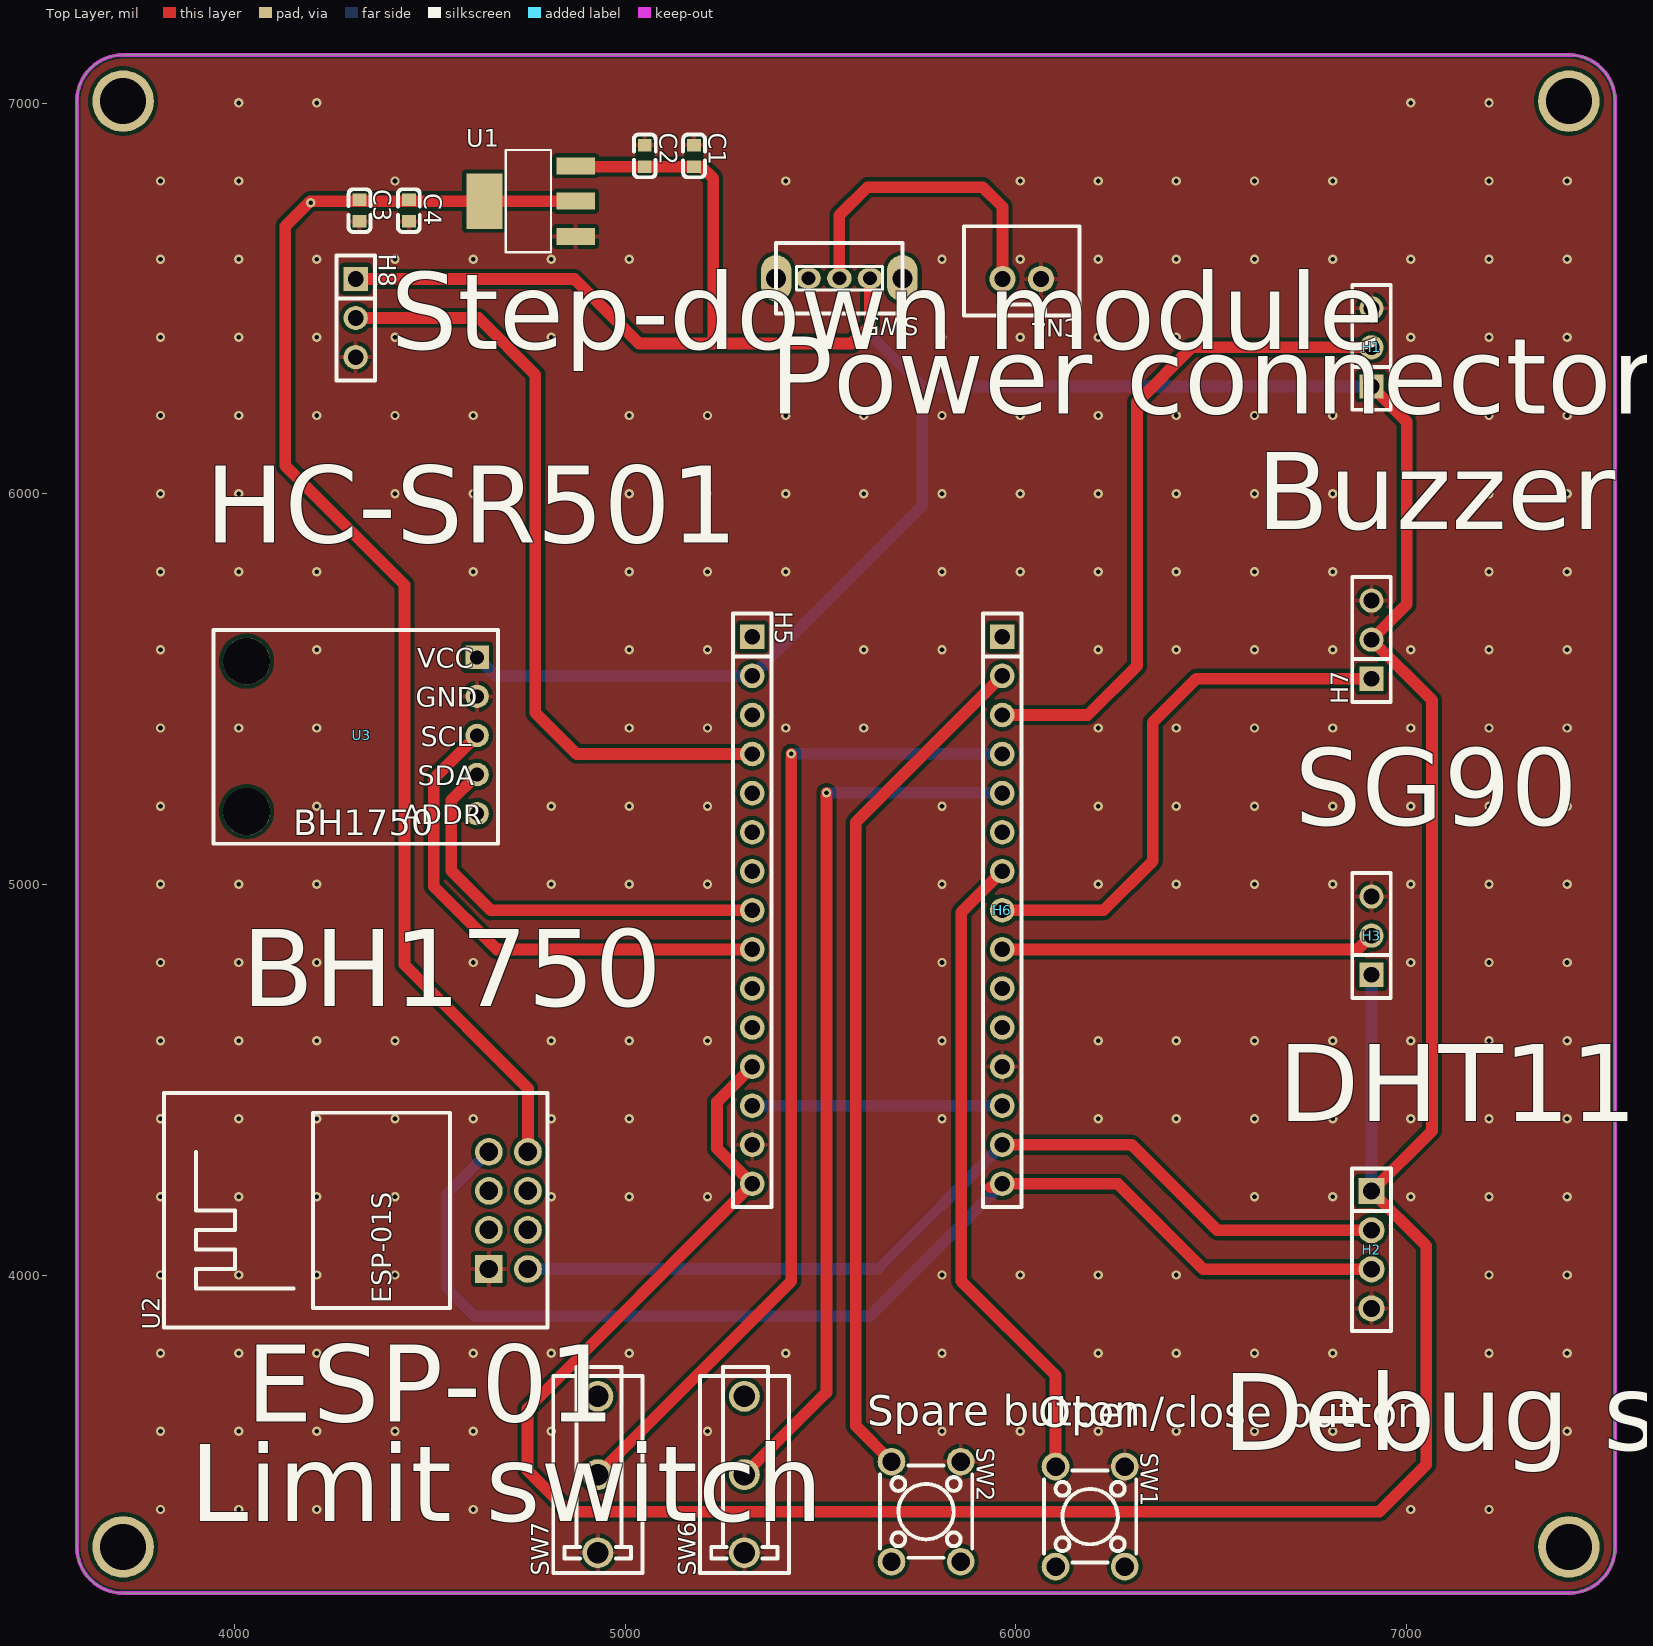
[diagram p0: Top Layer view]
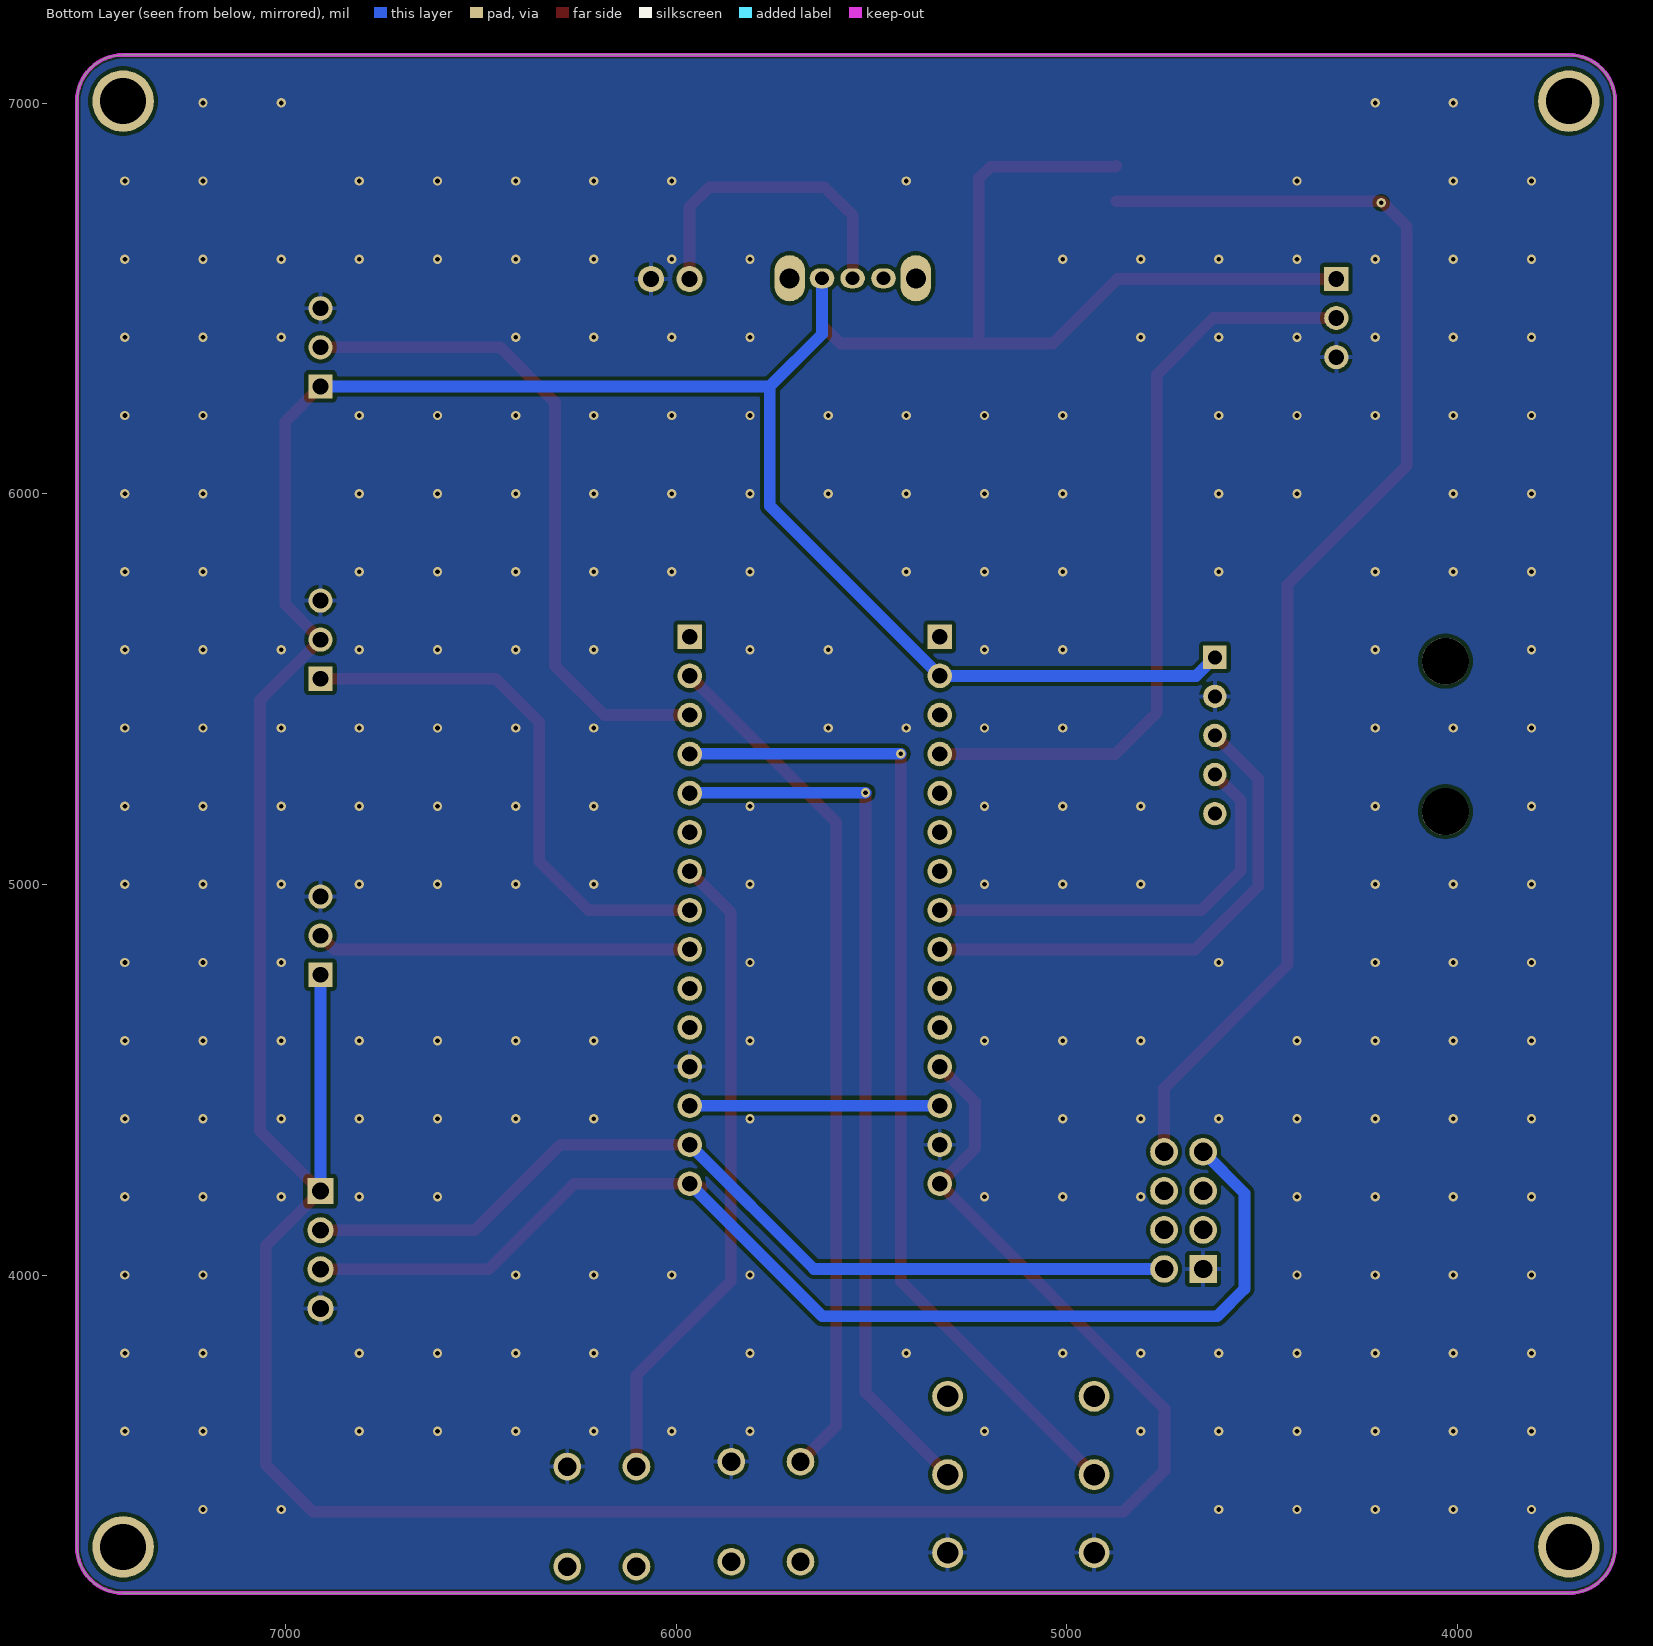
[diagram p1: Bottom Layer view, seen from below]
# Altium PCB MISC89126.pcbdoc
Units mil, origin at the board's own origin, x right, y up, seen from the top; angles counter-clockwise.
Board outline 3937.01 x 3937.01 mil, 2 copper layers (Top Layer, Bottom Layer), stack 62.206 mil thick; 20 components, 28 nets, 98 pads, 246 vias.

## Layer stack, top to bottom
Top Solder Mask Layer: solder mask 0.394, Dk 3.3
Top Layer: signal copper 1.379
Dielectric1: surface 59.449, FR4, Dk 4.5
Bottom Layer: signal copper 1.378
Bottom Solder Mask Layer: solder mask 0.394, Dk 3.3

## Board outline
3714.61,7123.5 ccw(c3714.61,7005.39) 3596.5,7005.39 3596.5,3304.61 ccw(c3714.61,3304.61) 3714.61,3186.5 7415.39,3186.5 ccw(c7415.39,3304.61) 7533.5,3304.61 7533.5,7005.39 ccw(c7415.39,7005.39) 7415.39,7123.5 3714.61,7123.5

## Design rules (kind name [scope] priority, off if disabled: settings)
BoardOutlineClearance copperThickness2oz_1 [All] p2 off: genericclearance=7.99 ignorepadtopadclearanceinfootprint=FALSE except(0: Arc-SplitContinuation Track-SplitContinuation SMDPad-SplitContinuation THPad-SplitContinuation Via-SplitContinuation Fill-SplitContinuation Region-SplitContinuation Poly-SplitContinuation Text-SplitContinuation Hole-SplitContinuation; 5.98: Arc-CutoutEdge Track-CutoutEdge SMDPad-CutoutEdge THPad-CutoutEdge Via-CutoutEdge Text-CutoutEdge; 6.9: Hole-OutlineEdge Hole-CutoutEdge; 10: Poly-OutlineEdge Poly-CutoutEdge; 11.81: Arc-OutlineEdge Track-OutlineEdge SMDPad-OutlineEdge THPad-OutlineEdge Via-OutlineEdge Fill-OutlineEdge Region-OutlineEdge Text-OutlineEdge Fill-CutoutEdge Region-CutoutEdge)
BoardOutlineClearance Plane_innerPlane_1 [All] p4 off: genericclearance=4.02 ignorepadtopadclearanceinfootprint=FALSE except(0: Arc-SplitContinuation Track-SplitContinuation SMDPad-SplitContinuation THPad-SplitContinuation Via-SplitContinuation Fill-SplitContinuation Region-SplitContinuation Poly-SplitContinuation Text-SplitContinuation Hole-SplitContinuation; 5.98: Arc-CutoutEdge Track-CutoutEdge SMDPad-CutoutEdge THPad-CutoutEdge Via-CutoutEdge Text-CutoutEdge; 6.9: Hole-OutlineEdge Hole-CutoutEdge; 10: Poly-OutlineEdge Poly-CutoutEdge; 11.81: Arc-OutlineEdge Track-OutlineEdge SMDPad-OutlineEdge THPad-OutlineEdge Via-OutlineEdge Fill-OutlineEdge Region-OutlineEdge Text-OutlineEdge Fill-CutoutEdge Region-CutoutEdge)
BoardOutlineClearance Copper_copperRegion_1 [All] p6 off: genericclearance=4.02 ignorepadtopadclearanceinfootprint=FALSE except(0: Arc-SplitContinuation Track-SplitContinuation SMDPad-SplitContinuation THPad-SplitContinuation Via-SplitContinuation Fill-SplitContinuation Region-SplitContinuation Poly-SplitContinuation Text-SplitContinuation Hole-SplitContinuation; 5.98: Arc-CutoutEdge Track-CutoutEdge SMDPad-CutoutEdge THPad-CutoutEdge Via-CutoutEdge Text-CutoutEdge; 6.9: Hole-OutlineEdge Hole-CutoutEdge; 10: Poly-OutlineEdge Poly-CutoutEdge; 11.81: Arc-OutlineEdge Track-OutlineEdge SMDPad-OutlineEdge THPad-OutlineEdge Via-OutlineEdge Fill-OutlineEdge Region-OutlineEdge Text-OutlineEdge Fill-CutoutEdge Region-CutoutEdge)
BoardOutlineClearance Copper_copperRegion_copperThickness1oz_1 [All] p8 off: genericclearance=4.02 ignorepadtopadclearanceinfootprint=FALSE except(0: Arc-SplitContinuation Track-SplitContinuation SMDPad-SplitContinuation THPad-SplitContinuation Via-SplitContinuation Fill-SplitContinuation Region-SplitContinuation Poly-SplitContinuation Text-SplitContinuation Hole-SplitContinuation; 5.98: Arc-CutoutEdge Track-CutoutEdge SMDPad-CutoutEdge THPad-CutoutEdge Via-CutoutEdge Text-CutoutEdge; 6.9: Hole-OutlineEdge Hole-CutoutEdge; 10: Poly-OutlineEdge Poly-CutoutEdge; 11.81: Arc-OutlineEdge Track-OutlineEdge SMDPad-OutlineEdge THPad-OutlineEdge Via-OutlineEdge Fill-OutlineEdge Region-OutlineEdge Text-OutlineEdge Fill-CutoutEdge Region-CutoutEdge)
BoardOutlineClearance Copper_copperRegion_Copper_copperRegion_1 [All] p10 off: genericclearance=4.02 ignorepadtopadclearanceinfootprint=FALSE except(0: Arc-SplitContinuation Track-SplitContinuation SMDPad-SplitContinuation THPad-SplitContinuation Via-SplitContinuation Fill-SplitContinuation Region-SplitContinuation Poly-SplitContinuation Text-SplitContinuation Hole-SplitContinuation; 5.98: Arc-CutoutEdge Track-CutoutEdge SMDPad-CutoutEdge THPad-CutoutEdge Via-CutoutEdge Text-CutoutEdge; 6.9: Hole-OutlineEdge Hole-CutoutEdge; 10: Poly-OutlineEdge Poly-CutoutEdge; 11.81: Arc-OutlineEdge Track-OutlineEdge SMDPad-OutlineEdge THPad-OutlineEdge Via-OutlineEdge Fill-OutlineEdge Region-OutlineEdge Text-OutlineEdge Fill-CutoutEdge Region-CutoutEdge)
BoardOutlineClearance copperThickness1oz_1 [All] p12: genericclearance=4.02 ignorepadtopadclearanceinfootprint=FALSE except(0: Arc-SplitContinuation Track-SplitContinuation SMDPad-SplitContinuation THPad-SplitContinuation Via-SplitContinuation Fill-SplitContinuation Region-SplitContinuation Poly-SplitContinuation Text-SplitContinuation Hole-SplitContinuation; 5.98: Arc-CutoutEdge Track-CutoutEdge SMDPad-CutoutEdge THPad-CutoutEdge Via-CutoutEdge Text-CutoutEdge; 6.9: Hole-OutlineEdge Hole-CutoutEdge; 10: Poly-OutlineEdge Poly-CutoutEdge; 11.81: Arc-OutlineEdge Track-OutlineEdge SMDPad-OutlineEdge THPad-OutlineEdge Via-OutlineEdge Fill-OutlineEdge Region-OutlineEdge Text-OutlineEdge Fill-CutoutEdge Region-CutoutEdge)
Clearance copperThickness2oz [All] p1 off: gap=7.99 ignorepadtopadclearanceinfootprint=FALSE except(5.98: SMDPad-Track SMDPad-SMDPad THPad-Track SMDPad-THPad THPad-THPad Track-Via SMDPad-Via THPad-Via Via-Via Fill-SMDPad Region-SMDPad Fill-THPad Region-THPad Fill-Via Region-Via Fill-Fill Fill-Region Region-Region Arc-Track Arc-SMDPad Arc-THPad Arc-Via Fill-Arc Region-Arc Arc-Arc Text-Track SMDPad-Text Text-THPad Text-Via Fill-Text Region-Text Arc-Text Text-Text; 6.9: Hole-Track Hole-SMDPad Hole-THPad Hole-Via Fill-Hole Region-Hole Hole-Arc Hole-Text; 10: Poly-Track Poly-SMDPad Poly-THPad Poly-Via Poly-Fill Poly-Region Poly-Poly Poly-Arc Poly-Text Poly-Hole; 11.81: Fill-Track Region-Track)
Clearance Plane_innerPlane [All] p3 off: gap=4.02 ignorepadtopadclearanceinfootprint=FALSE except(5.98: SMDPad-Track SMDPad-SMDPad THPad-Track SMDPad-THPad THPad-THPad Track-Via SMDPad-Via THPad-Via Via-Via Fill-SMDPad Region-SMDPad Fill-THPad Region-THPad Fill-Via Region-Via Fill-Fill Fill-Region Region-Region Arc-Track Arc-SMDPad Arc-THPad Arc-Via Fill-Arc Region-Arc Arc-Arc Text-Track SMDPad-Text Text-THPad Text-Via Fill-Text Region-Text Arc-Text Text-Text; 6.9: Hole-Track Hole-SMDPad Hole-THPad Hole-Via Fill-Hole Region-Hole Hole-Arc Hole-Text; 10: Poly-Track Poly-SMDPad Poly-THPad Poly-Via Poly-Fill Poly-Region Poly-Poly Poly-Arc Poly-Text Poly-Hole; 11.81: Fill-Track Region-Track)
Clearance Copper_copperRegion [All] p5 off: gap=4.02 ignorepadtopadclearanceinfootprint=FALSE except(5.98: SMDPad-Track SMDPad-SMDPad THPad-Track SMDPad-THPad THPad-THPad Track-Via SMDPad-Via THPad-Via Via-Via Fill-SMDPad Region-SMDPad Fill-THPad Region-THPad Fill-Via Region-Via Fill-Fill Fill-Region Region-Region Arc-Track Arc-SMDPad Arc-THPad Arc-Via Fill-Arc Region-Arc Arc-Arc Text-Track SMDPad-Text Text-THPad Text-Via Fill-Text Region-Text Arc-Text Text-Text; 6.9: Hole-Track Hole-SMDPad Hole-THPad Hole-Via Fill-Hole Region-Hole Hole-Arc Hole-Text; 10: Poly-Track Poly-SMDPad Poly-THPad Poly-Via Poly-Fill Poly-Region Poly-Poly Poly-Arc Poly-Text Poly-Hole; 11.81: Fill-Track Region-Track)
Clearance Copper_copperRegion_copperThickness1oz [All] p7 off: gap=4.02 ignorepadtopadclearanceinfootprint=FALSE except(5.98: SMDPad-Track SMDPad-SMDPad THPad-Track SMDPad-THPad THPad-THPad Track-Via SMDPad-Via THPad-Via Via-Via Fill-SMDPad Region-SMDPad Fill-THPad Region-THPad Fill-Via Region-Via Fill-Fill Fill-Region Region-Region Arc-Track Arc-SMDPad Arc-THPad Arc-Via Fill-Arc Region-Arc Arc-Arc Text-Track SMDPad-Text Text-THPad Text-Via Fill-Text Region-Text Arc-Text Text-Text; 6.9: Hole-Track Hole-SMDPad Hole-THPad Hole-Via Fill-Hole Region-Hole Hole-Arc Hole-Text; 10: Poly-Track Poly-SMDPad Poly-THPad Poly-Via Poly-Fill Poly-Region Poly-Poly Poly-Arc Poly-Text Poly-Hole; 11.81: Fill-Track Region-Track)
Clearance Copper_copperRegion_Copper_copperRegion [All] p9 off: gap=4.02 ignorepadtopadclearanceinfootprint=FALSE except(5.98: SMDPad-Track SMDPad-SMDPad THPad-Track SMDPad-THPad THPad-THPad Track-Via SMDPad-Via THPad-Via Via-Via Fill-SMDPad Region-SMDPad Fill-THPad Region-THPad Fill-Via Region-Via Fill-Fill Fill-Region Region-Region Arc-Track Arc-SMDPad Arc-THPad Arc-Via Fill-Arc Region-Arc Arc-Arc Text-Track SMDPad-Text Text-THPad Text-Via Fill-Text Region-Text Arc-Text Text-Text; 6.9: Hole-Track Hole-SMDPad Hole-THPad Hole-Via Fill-Hole Region-Hole Hole-Arc Hole-Text; 10: Poly-Track Poly-SMDPad Poly-THPad Poly-Via Poly-Fill Poly-Region Poly-Poly Poly-Arc Poly-Text Poly-Hole; 11.81: Fill-Track Region-Track)
Clearance copperThickness1oz [All] p11: gap=4.02 ignorepadtopadclearanceinfootprint=FALSE except(5.98: SMDPad-Track SMDPad-SMDPad THPad-Track SMDPad-THPad THPad-THPad Track-Via SMDPad-Via THPad-Via Via-Via Fill-SMDPad Region-SMDPad Fill-THPad Region-THPad Fill-Via Region-Via Fill-Fill Fill-Region Region-Region Arc-Track Arc-SMDPad Arc-THPad Arc-Via Fill-Arc Region-Arc Arc-Arc Text-Track SMDPad-Text Text-THPad Text-Via Fill-Text Region-Text Arc-Text Text-Text; 6.9: Hole-Track Hole-SMDPad Hole-THPad Hole-Via Fill-Hole Region-Hole Hole-Arc Hole-Text; 10: Poly-Track Poly-SMDPad Poly-THPad Poly-Via Poly-Fill Poly-Region Poly-Poly Poly-Arc Poly-Text Poly-Hole; 11.81: Fill-Track Region-Track)
DiffPairsRouting differentialPair [All] p1: maxlimit=6 minlimit=6 mostfreqgap=6 toplayer_minwidth=5 toplayer_prefwidth=10 toplayer_maxwidth=100 toplayer_mingap=6 toplayer_prefgap=6 toplayer_maxgap=6 bottomlayer_minwidth=5 bottomlayer_prefwidth=10 bottomlayer_maxwidth=100 bottomlayer_mingap=6 bottomlayer_prefgap=6 bottomlayer_maxgap=6 maxuncoupledlength=10
HoleToHoleClearance otherClearance [All] p1: gap=11.81 allowstackedmicrovias=TRUE
Length netLength [All] p1: minlimit=0 maxlimit=0
PasteMaskExpansion pasteMaskExpansion [All] p1: expansion=0
PlaneConnect innerPlane [All] p1: planeconnectstyle=Relief reliefexpansion=20 reliefentries=4 reliefconductorwidth=10 reliefairgap=10
PolygonConnect copperRegion_copperThickness1oz [All] p1 off: connectstyle=Relief reliefconductorwidth=10 reliefentries=4 polygonreliefangle="90 Angle" airgapwidth=10 via.connectstyle=Relief via.reliefconductorwidth=10 via.reliefentries=4 via.polygonreliefangle="90 Angle" via.airgapwidth=10
PolygonConnect copperRegion_Copper_copperRegion [All] p2 off: connectstyle=Relief reliefconductorwidth=10 reliefentries=4 polygonreliefangle="90 Angle" airgapwidth=10 via.connectstyle=Relief via.reliefconductorwidth=10 via.reliefentries=4 via.polygonreliefangle="90 Angle" via.airgapwidth=10
PolygonConnect copperRegion [All] p3: connectstyle=Relief reliefconductorwidth=10 reliefentries=4 polygonreliefangle="90 Angle" airgapwidth=10 via.connectstyle=Relief via.reliefconductorwidth=10 via.reliefentries=4 via.polygonreliefangle="90 Angle" via.airgapwidth=10
RoutingVias viaSize [All] p1: holewidth=12.01 width=24.02 viastyle="Through Hole" minholewidth=11.81 minwidth=19.68 maxholewidth=248.03 maxwidth=393.7
SolderMaskExpansion solderMaskExpansion [IsVia] p1: expansion=-1000 istentingtop=TRUE
SolderMaskExpansion solderMaskExpansion [All] p2: expansion=2 istentingtop=FALSE
Width copperThickness2oz_2 [All] p1 off: maxlimit=100 minlimit=8 preferedwidth=10
Width copperThickness1oz_2 [All] p2: maxlimit=100 minlimit=5 preferedwidth=10

## Components (designator, comment, footprint, x,y, rotation, side; value= is the part's Value field where it differs from the comment)
C1 "100nF" C0603 5176.19,6864.94 r270 top
C2 "10uF" C0603 5050,6865 r270 top
C3 "10uF" C0603 4320,6725 r90 top
C4 "100nF" C0603 4446.13,6724.94 r90 top
CN4 "XH2.54*2P_through-hole" CONN-TH_2P-P2.50-XH2.54-2P 6015,6550 r180 top
H1 "" HDR-TH_3P-P2.54-V-F 6910,6375 r90 top
H2 "" HDR-TH_4P-P2.54-V-F 6910,4065.31 r270 top
H3 "" HDR-TH_3P-P2.54-V-F 6910,4869.28 r90 top
H5 "" HDR-TH_15P-P2.54-V-F-1 5325,4934.06 r270 top
H6 "" HDR-TH_15P-P2.54-V-F-1 5965,4934.06 r270 top
H7 "" HDR-TH_3P-P2.54-V-F 6910,5626.91 r90 top
H8 "" HDR-TH_3P-P2.54-V-F 4310,6450 r270 top
SW1 "" SW-TH_4P-L6.0-W6.0-P4.50-LS6.5 6189.85,3382.47 r270 top
SW2 "" SW-TH_4P-L6.0-W6.0-P4.50-LS6.5 5770,3395 r270 top
SW5 "" 拨动开关 5553,6551.78 r180 top
SW6 "DM1-12UP-1" SW-TH_DM1-12UP-1 5305,3490 r90 top
SW7 "DM1-12UP-1" SW-TH_DM1-12UP-1 4930,3490 r90 top
U1 "AMS1117-3.3" SOT-223-3_L6.5-W3.4-P2.30-LS7.0-BR 4756.15,6749.1 r0 top
U2 "ESP-01S" WIFIM-TH_ESP-01S 4701,4166.01 r90 top
U3 "" BH1750光照传感器 4360.83,5371.61 r0 top

## Footprints (in the part's own frame and the unit in brackets; to place one, negate y for a bottom-side part, rotate by r counter-clockwise, add the part's x,y. Pads: shape width x height; smd on the part's side, far side on the other; paste and mask are expansions set on the pad)
BH1750光照传感器 [mil]
  rect 60x60 hole 36: 1(260,210)
  round 60 hole 36: 2(260,110) 3(260,10) 4(260,-90) 5(260,-190)
  round 120 hole 120 unplated: ""(-330,-185) ""(-330,200)
  silkscreen extent -415,-267 313,280
C0603 [mm]
  rect 0.8x0.9 smd: 1(-0.7,0) 2(0.7,0)
  silkscreen extent -1.39,-0.71 1.39,0.71
CONN-TH_2P-P2.50-XH2.54-2P [mm]
  round 1.7 hole 1.05 paste+0 mask+0.05: 1(1.25,0) 2(-1.25,0)
  silkscreen extent -3.75,-3.42 3.75,2.37
HDR-TH_3P-P2.54-V-F [mil]
  rect 62x62 hole 40.16: 1(-100,0)
  round 62 hole 40.16: 2(0,0) 3(100,0)
  silkscreen extent -160,-49 160,49
HDR-TH_4P-P2.54-V-F [mm]
  rect 1.7x1.7 hole 1.1: 1(-3.81,0)
  round 1.7 hole 1.1: 2(-1.27,0) 3(1.27,0) 4(3.81,0)
  silkscreen extent -5.29,-1.27 5.29,1.27
HDR-TH_15P-P2.54-V-F-1 [mm]
  rect 1.6x1.575 hole 1: 1(-17.78,0)
  round 1.6 hole 1: 2(-15.24,0) 3(-12.7,0) 4(-10.16,0) 5(-7.62,0) 6(-5.08,0) 7(-2.54,0) 8(0,0) 9(2.54,0) 10(5.08,0) 11(7.62,0) 12(10.16,0) 13(12.7,0) 14(15.24,0) 15(17.78,0)
  silkscreen extent -19.3,-1.25 19.3,1.25
SOT-223-3_L6.5-W3.4-P2.30-LS7.0-BR [mm]
  rect 2.5x1.1 smd: 1(2.97,-2.3) 2(2.97,0) 3(2.97,2.3)
  rect 2.34x3.6 smd: 4(-2.97,0)
  silkscreen extent -1.57,-3.33 1.37,3.33
SW-TH_4P-L6.0-W6.0-P4.50-LS6.5 [mm]
  round 1.8 hole 1.2: 1(-3.25,2.25) 2(3.25,2.25) 3(-3.25,-2.25) 4(3.25,-2.25)
  silkscreen extent -3,-3 3,3
SW-TH_DM1-12UP-1 [mm]
  round 2 hole 1.4: 1(-5.08,0) 2(0,0) 3(5.08,0)
  silkscreen extent -6.4,-2.9 7,2.9
WIFIM-TH_ESP-01S [mm]
  rect 1.8x1.8 hole 1.2: 1(-3.81,1.27)
  round 1.8 hole 1.2: 2(-1.27,1.27) 3(1.27,1.27) 4(3.81,1.27) 5(3.81,-1.27) 6(1.27,-1.27) 7(-1.27,-1.27) 8(-3.81,-1.27)
  silkscreen extent -7.62,-2.54 7.62,22.4
拨动开关 [mil]
  oval 63x51.2 hole 35.4 paste+0 mask+2: 1(-73.4,0) 2(5,0) 3(84,0)
  oval 78.7x118.1 hole 51.2 paste+0 mask+2: 4(166.7,0) 5(-156.1,0)
  silkscreen extent -156,-90 167,90

## Free pads (board coordinates)
  round 157.48 hole 118.11: 1(3714.61,7005.39) 1(3714.61,3304.61) 1(7415.39,7005.39) 1(7415.39,3304.61)

## Via types
v1: diameter 24.02, hole 12, Top Layer to Bottom Layer, 246 vias

## Nets (pads, with @x,y where several pads share a name; then routed paths per layer and width w, separated by ;. In a path a pad name is that pad's centre, name@x,y a point inside that pad or via, vN(x,y) a via of type N, cw(c..) or ccw(c..) an arc to the next point about the centre after c; other vN are vias at no path point)
$1N17196: CN4.1 SW5.2 | length 814.1
  Top Layer w30: SW5.2 5548,6713 5620,6785 5915,6785 5965.78,6734.22 CN4.1
+5V: C1.2 C2.2 H1.1 H2.1 H3.1 H5.2 H5.12 H5.15 H7.2 H8.1 SW5.1 U1.3 U3.1 | length 12754
  Top Layer w30: H8.1 4870,6550 5035,6385 5225,6385 ; U1.3 4875.29,6837.44 C2.2 ; C2.2@5050.06,6837.38 C1.2 5195,6837.38 5225,6807.38 5225,6385 ; H5.12 5235,4444.06 5235,4324.06 H5.15 4750,3659.06 4750,3500 4855,3395 6930,3395 7050,3515 7050,4075.31 H2.1 7065,4370.31 7065,5471.91 H7.2 7000,5716.91 7000,6185 H1.1 ; SW5.1 5626.4,6431.4 5580,6385 5225,6385
  Bottom Layer w30: U3.1 4668.38,5534.06 H5.2 5760,5969.06 5760,6275 ; SW5.1 5626.4,6408.6 5760,6275 ; H2.1 H3.1 ; H1.1 5760,6275
A0: H5.4 H8.2 | length 1983.9
  Top Layer w30: H8.2 4625,6450 4770,6305 4770,5440 4875.94,5334.06 H5.4
A1: H5.5
A2: H5.6
A3: H5.7
A4: H5.8 U3.4 | length 1085.7
  Top Layer w30: U3.4 4555,5215.78 4555,5035 4655.94,4934.06 H5.8
A5: H5.9 U3.3 | length 1314.2
  Top Layer w30: U3.3 4510,5270.78 4510,4995 4670.94,4834.06 H5.9
A6: H5.10
A7: H5.11
D2: H6.11
D3: H6.10
D4: H3.2 H6.9 | length 959.6
  Top Layer w30: H6.9 6874.77,4834.06 H3.2
D5: H6.8 H7.1 | length 1398.5
  Top Layer w30: H6.8 6224.06,4934.06 6350,5060 6350,5415 6461.91,5526.91 H7.1
D6: H6.7 SW1.3 | length 1667.1
  Top Layer w30: H6.7 5860,4929.06 5860,3985 6101.27,3743.73 SW1.3
D7: H6.6
D8: H6.5 SW6.2 | length 2282.4
  Top Layer w30: SW6.2 5515,3700 v1(5515,5235)
  Bottom Layer w30: v1(5515,5235) 5964.06,5235 H6.5
D9: H6.4 SW7.2 | length 2590.4
  Top Layer w30: SW7.2 5425,3985 v1(5425,5335)
  Bottom Layer w30: v1(5425,5335) 5964.06,5335 H6.4
D10: H1.2 H6.3 | length 1730.2
  Top Layer w30: H6.3 6184.06,5434.06 6310,5560 6310,6235 6450,6375 H1.2
D11: H6.2 SW2.3 | length 2204.3
  Top Layer w30: SW2.3 5590,3614.37 5590,5159.06 H6.2
D12: H6.1
D13: H5.1
GND: C1.1 C2.1 C3.1 C4.1 CN4.2 H1.3 H2.4 H3.3 H5.14 H6.12 H7.3 H8.3 SW1.1 SW2.1 SW6.1 SW7.1 U1.1 U2.1 U3.2
  other v1: 3810.6,3400.6 4010.6,3400.6 4210.6,3400.6 4410.6,3400.6 4610.6,3400.6 7010.6,3400.6 7210.6,3400.6 3810.6,3600.6 4010.6,3600.6 4210.6,3600.6 4410.6,3600.6 4610.6,3600.6 4810.6,3600.6 5210.6,3600.6 5810.6,3600.6 6010.6,3600.6 6210.6,3600.6 6410.6,3600.6 6610.6,3600.6 6810.6,3600.6 7210.6,3600.6 7410.6,3600.6 3810.6,3800.6 4010.6,3800.6 4210.6,3800.6 4410.6,3800.6 4610.6,3800.6 4810.6,3800.6 5010.6,3800.6 5410.6,3800.6 5810.6,3800.6 6210.6,3800.6 6410.6,3800.6 6610.6,3800.6 6810.6,3800.6 7210.6,3800.6 7410.6,3800.6 3810.6,4000.6 4010.6,4000.6 4210.6,4000.6 4410.6,4000.6 5810.6,4000.6 6010.6,4000.6 6210.6,4000.6 6410.6,4000.6 7210.6,4000.6 7410.6,4000.6 3810.6,4200.6 4010.6,4200.6 4210.6,4200.6 4410.6,4200.6 4810.6,4200.6 5010.6,4200.6 5210.6,4200.6 6610.6,4200.6 6810.6,4200.6 7010.6,4200.6 7210.6,4200.6 7410.6,4200.6 3810.6,4400.6 4010.6,4400.6 4210.6,4400.6 4410.6,4400.6 4610.6,4400.6 4810.6,4400.6 5010.6,4400.6 5810.6,4400.6 6210.6,4400.6 6410.6,4400.6 6610.6,4400.6 6810.6,4400.6 7010.6,4400.6 7210.6,4400.6 7410.6,4400.6 3810.6,4600.6 4010.6,4600.6 4210.6,4600.6 4410.6,4600.6 4810.6,4600.6 5010.6,4600.6 5210.6,4600.6 5810.6,4600.6 6210.6,4600.6 6410.6,4600.6 6610.6,4600.6 6810.6,4600.6 7010.6,4600.6 7210.6,4600.6 7410.6,4600.6 3810.6,4800.6 4010.6,4800.6 4210.6,4800.6 4610.6,4800.6 5810.6,4800.6 7010.6,4800.6 7210.6,4800.6 7410.6,4800.6 3810.6,5000.6 4010.6,5000.6 4210.6,5000.6 4810.6,5000.6 5010.6,5000.6 5210.6,5000.6 5810.6,5000.6 6210.6,5000.6 6410.6,5000.6 6610.6,5000.6 6810.6,5000.6 7010.6,5000.6 7210.6,5000.6 7410.6,5000.6 3810.6,5200.6 4210.6,5200.6 4810.6,5200.6 5010.6,5200.6 5210.6,5200.6 5810.6,5200.6 6210.6,5200.6 6410.6,5200.6 6610.6,5200.6 6810.6,5200.6 7010.6,5200.6 7210.6,5200.6 7410.6,5200.6 3810.6,5400.6 4010.6,5400.6 4210.6,5400.6 5010.6,5400.6 5210.6,5400.6 5410.6,5400.6 5610.6,5400.6 6210.6,5400.6 6410.6,5400.6 6610.6,5400.6 6810.6,5400.6 7010.6,5400.6 7210.6,5400.6 7410.6,5400.6 3810.6,5600.6 4210.6,5600.6 5010.6,5600.6 5210.6,5600.6 5610.6,5600.6 5810.6,5600.6 6210.6,5600.6 6410.6,5600.6 6610.6,5600.6 6810.6,5600.6 7010.6,5600.6 7210.6,5600.6 7410.6,5600.6 3810.6,5800.6 4010.6,5800.6 4210.6,5800.6 4610.6,5800.6 5010.6,5800.6 5210.6,5800.6 5410.6,5800.6 5810.6,5800.6 6010.6,5800.6 6210.6,5800.6 6410.6,5800.6 6610.6,5800.6 6810.6,5800.6 7210.6,5800.6 7410.6,5800.6 3810.6,6000.6 4010.6,6000.6 4410.6,6000.6 4610.6,6000.6 5010.6,6000.6 5210.6,6000.6 5410.6,6000.6 5610.6,6000.6 5810.6,6000.6 6010.6,6000.6 6210.6,6000.6 6410.6,6000.6 6610.6,6000.6 6810.6,6000.6 7210.6,6000.6 7410.6,6000.6 3810.6,6200.6 4010.6,6200.6 4210.6,6200.6 4410.6,6200.6 4610.6,6200.6 5010.6,6200.6 5210.6,6200.6 5410.6,6200.6 5610.6,6200.6 5810.6,6200.6 6010.6,6200.6 6210.6,6200.6 6410.6,6200.6 6610.6,6200.6 6810.6,6200.6 7210.6,6200.6 7410.6,6200.6 3810.6,6400.6 4010.6,6400.6 4210.6,6400.6 4410.6,6400.6 4610.6,6400.6 4810.6,6400.6 5810.6,6400.6 6010.6,6400.6 6210.6,6400.6 6410.6,6400.6 7010.6,6400.6 7210.6,6400.6 7410.6,6400.6 3810.6,6600.6 4010.6,6600.6 4210.6,6600.6 4410.6,6600.6 4610.6,6600.6 4810.6,6600.6 5010.6,6600.6 5810.6,6600.6 6010.6,6600.6 6210.6,6600.6 6410.6,6600.6 6610.6,6600.6 6810.6,6600.6 7010.6,6600.6 7210.6,6600.6 7410.6,6600.6 3810.6,6800.6 4010.6,6800.6 4410.6,6800.6 5410.6,6800.6 6010.6,6800.6 6210.6,6800.6 6410.6,6800.6 6610.6,6800.6 6810.6,6800.6 7210.6,6800.6 7410.6,6800.6 4010.6,7000.6 4210.6,7000.6 7010.6,7000.6 7210.6,7000.6
REF: H5.3
RST: H5.13 H6.13 | length 640
  Bottom Layer w30: H5.13 H6.13
RXD: H2.2 H6.14 U2.8 | length 2381.3
  Top Layer w30: H6.14 6295.94,4334.06 6514.69,4115.31 H2.2
  Bottom Layer w30: U2.8 5646.96,4016.01 H6.14
TXD: H2.3 H6.15 U2.4 | length 3050
  Top Layer w30: H6.15@5935,4225 H6.15@5965,4225 ; H6.15 6260.94,4234.06 6479.69,4015.31 H2.3
  Bottom Layer w30: U2.4 4545,4210.01 4545,3965 4615,3895 5625.94,3895 H6.15
VCC: C3.2 C4.2 U1.2 U1.4 U2.5 | length 3395.8
  Top Layer w30: U2.5 4751,4479 4435,4795 4435,5767.44 4130,6072.44 4130,6685 4194.1,6749.1 U1.4 U1.2
  other v1: 4195,6745
pads on no net: SW1.2 SW1.4 SW2.2 SW2.4 SW5.3 SW5.4 SW5.5 SW6.3 SW7.3 U2.2 U2.3 U2.6 U2.7 U3. U3.5

## Polygon pours and split planes (outlines as drawn)
GND on Bottom Layer (solid, remove dead copper, pour order 2): 3525,7245 3525,3080 7700,3080 7700,7245
GND on Top Layer (solid, remove dead copper, pour order 2): 3000,7415 3000,3000 7930,3000 7930,7415

## Keep-outs
Board Outline Layer:
  the board outline again, w10

## Silkscreen, mask and mechanical layers (free items; w line width, h text height)
Top Silkscreen Layer:
  text "Step-down module" at 4400,6370 h196.85
  text "Power connector" at 5370,6205 h196.85
  text "Buzzer" at 6616.81,5909.09 h196.85
  text "HC-SR501" at 3924.95,5874.25 h196.85
  text "SG90" at 6713.9,5151.46 h196.85
  text "BH1750" at 4018.3,4688.75 h196.85
  text "DHT11" at 6671.39,4394.13 h196.85
  text "ESP-01" at 4030,3625 h196.85
  text "Spare button" at 5620,3615 h78.74
  text "Open/close button" at 6057.52,3610.63 h78.74
  text "Debug serial port" at 6529.27,3551.57 h196.85
  text "Limit switch" at 3885,3370 h196.85